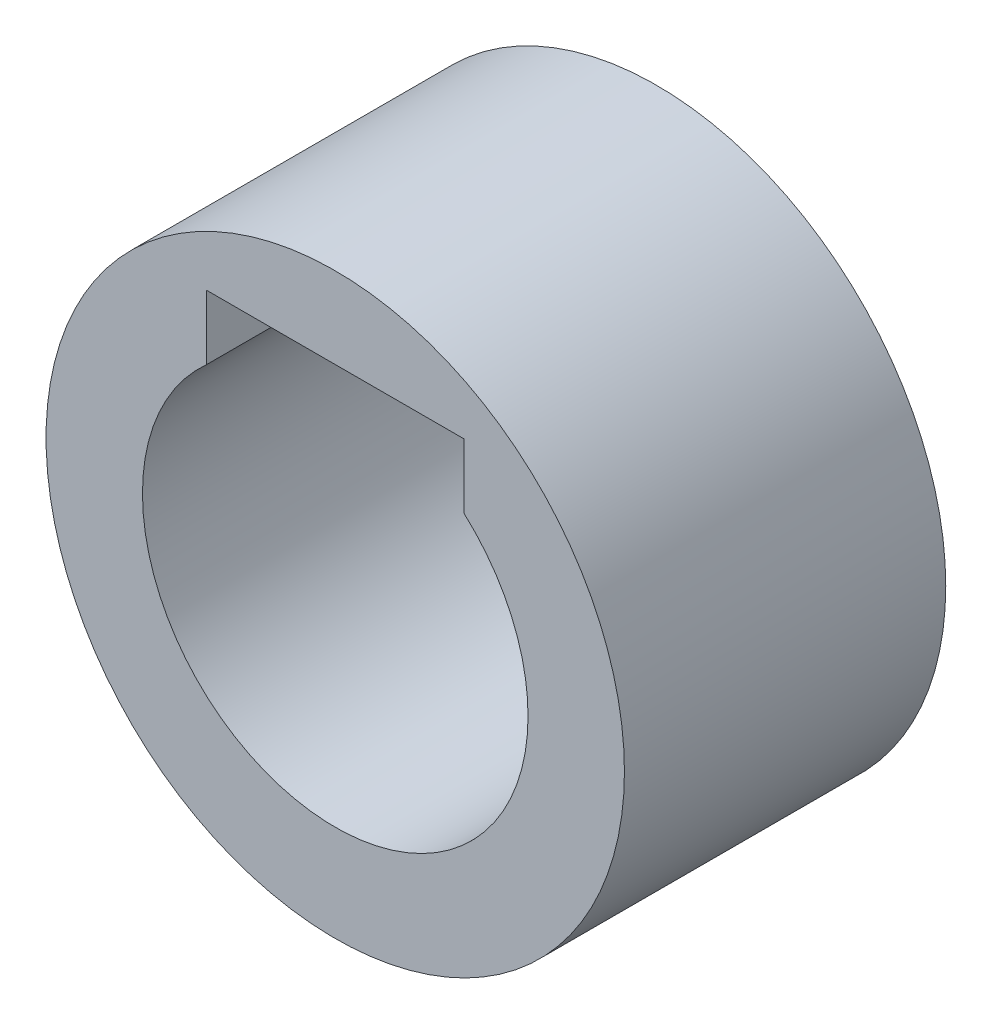
SolidWorks part; units mm, degrees
ref_plane "前视基准面" through (0, 0, 0) normal (0, 0, 1) x (1, 0, 0)
ref_plane "上视基准面" through (0, 0, 0) normal (0, 1, 0) x (1, 0, 0)
ref_plane "右视基准面" through (0, 0, 0) normal (1, 0, 0) x (0, 0, -1)
other "Configuration Table"
sketch "草图1" plane through (0, 0, 0) normal (0, 0, 1) x (1, 0, 0)
  line L0 (-4.2749, 6.3204) -> (3.7251, 6.3204)
  line L1 (-0.2749, -0.1517) -> (-0.2749, 8.8483) construction
  line L2 (-4.2749, 6.3204) -> (-4.2749, 4.3204)
  line L3 (3.7251, 6.3204) -> (3.7251, 4.3204)
  arc A0 (-4.2749, 4.3204) -> (3.7251, 4.3204) centre (-0.2749, -0.1517) ccw
  circle A1 centre (-0.2749, -0.1517) radius 9
  dimension "D1" = 12
  dimension "D2" = 18
  dimension "D3" = 8
extrude "凸台-拉伸1" add sketch "草图1" along normal blind 10
